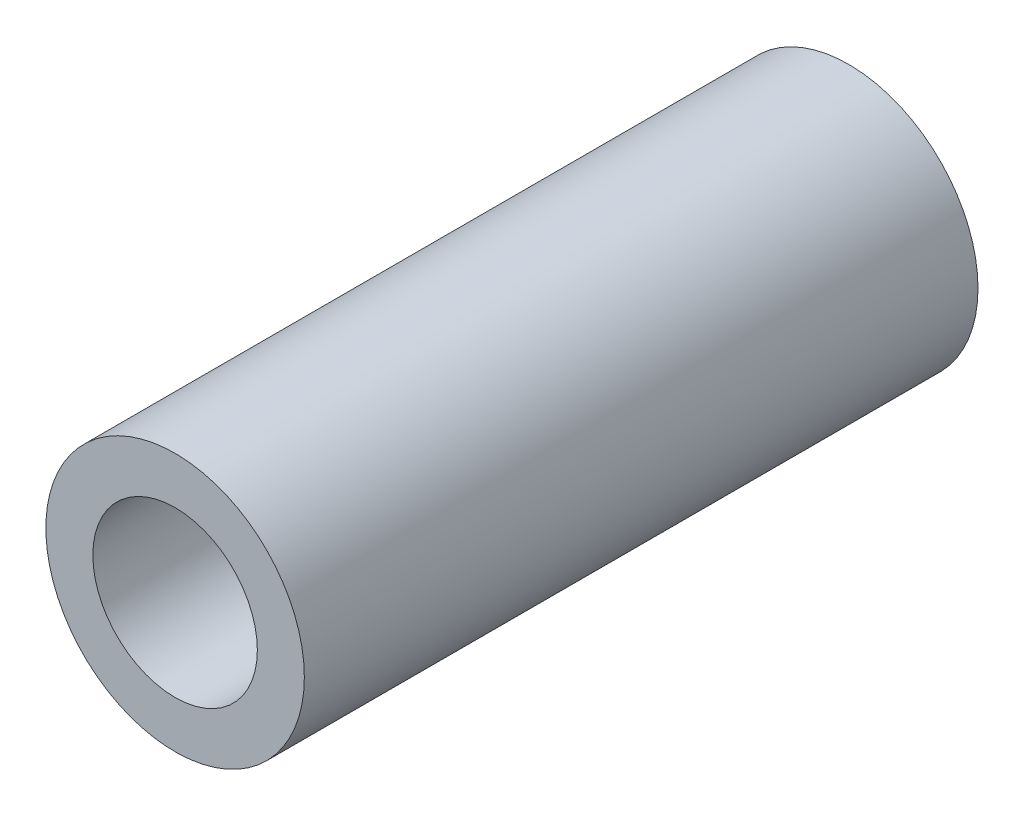
from build123d import *

# Parameters (mm, degrees)
SKETCH1_R           = 8.25
BOSS_EXTRUDE1_DEPTH = 43
SKETCH2_R           = 5.25
CUT_EXTRUDE1_DEPTH  = 100


with BuildPart() as part:
    # Sketch1 → Boss-Extrude1 (new body)
    with BuildSketch(Plane.XY):
        Circle(SKETCH1_R)
    extrude(amount=BOSS_EXTRUDE1_DEPTH)

    # Sketch2 → Cut-Extrude1 (cut)
    with BuildSketch(Plane.XY.offset(43)):
        Circle(SKETCH2_R)
    extrude(amount=-CUT_EXTRUDE1_DEPTH, mode=Mode.SUBTRACT)


solid = part.part
